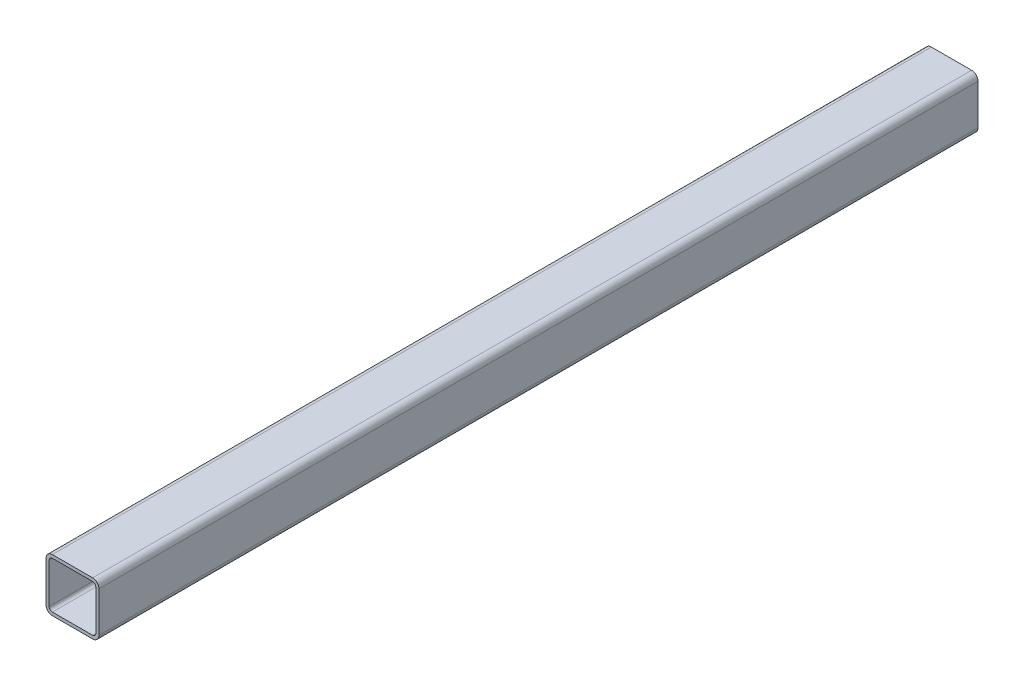
from build123d import *

# Parameters (mm, degrees)
GB_6728_1986_050_X_50_X_3_1_DEPTH = 830


with BuildPart() as part:
    # Sketch1 → Gb／6728-1986方形空心型钢 050 X 50 X 3(1) (new body)
    with BuildSketch(Plane.YX.offset(-415)):
        with BuildLine():
            Line((-19, -25), (19, -25))
            ThreePointArc((19, -25), (23.242640687, -23.242640687), (25, -19))
            Line((25, -19), (25, 19))
            ThreePointArc((25, 19), (23.242640687, 23.242640687), (19, 25))
            Line((19, 25), (-19, 25))
            ThreePointArc((-19, 25), (-23.242640687, 23.242640687), (-25, 19))
            Line((-25, 19), (-25, -19))
            ThreePointArc((-25, -19), (-23.242640687, -23.242640687), (-19, -25))
        make_face()
        with BuildLine():
            Line((-19, -22), (19, -22))
            ThreePointArc((19, -22), (21.121320344, -21.121320344), (22, -19))
            Line((22, -19), (22, 19))
            ThreePointArc((22, 19), (21.121320344, 21.121320344), (19, 22))
            Line((19, 22), (-19, 22))
            ThreePointArc((-19, 22), (-21.121320344, 21.121320344), (-22, 19))
            Line((-22, 19), (-22, -19))
            ThreePointArc((-22, -19), (-21.121320344, -21.121320344), (-19, -22))
        make_face(mode=Mode.SUBTRACT)
    extrude(amount=GB_6728_1986_050_X_50_X_3_1_DEPTH)


solid = part.part
